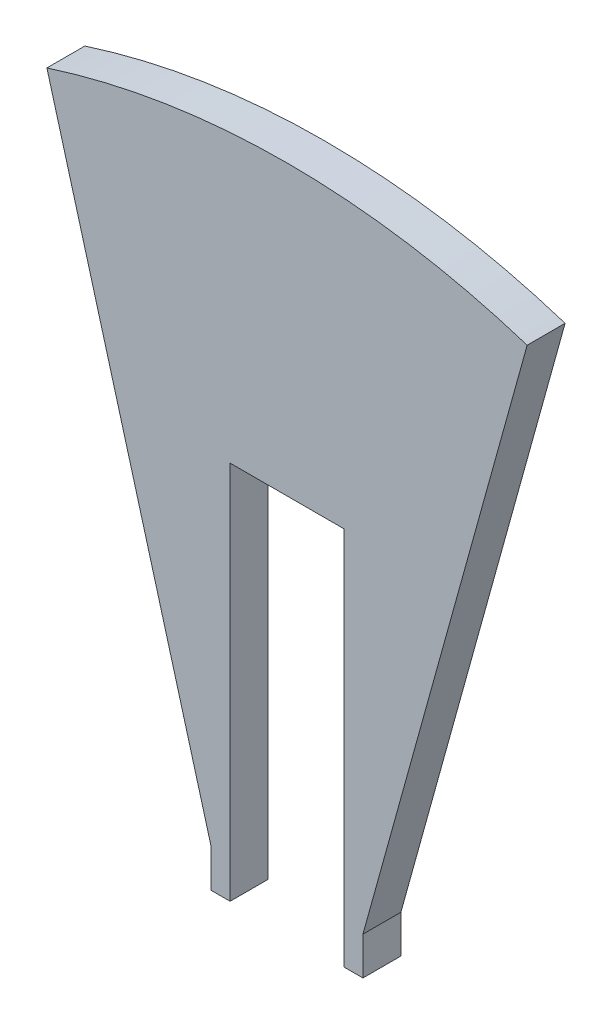
from build123d import *

# Parameters (mm, degrees)
BOSS_EXTRUDE1_DEPTH = 5
SKETCH2_W           = 30
SKETCH2_H           = 200
CUT_EXTRUDE1_DEPTH  = 10


with BuildPart() as part:
    # Sketch1 → Boss-Extrude1 (new, symmetric)
    with BuildSketch(Plane.XY):
        with BuildLine():
            Line((-63.274211694, 196.041766301), (-20, 40))
            Line((-20, 40), (-20, 30))
            Line((-20, 30), (20, 30))
            Line((20, 30), (20, 40))
            Line((20, 40), (63.274211694, 196.041766301))
            ThreePointArc((63.274211694, 196.041766301), (0, 206), (-63.274211694, 196.041766301))
        make_face()
    extrude(amount=BOSS_EXTRUDE1_DEPTH, both=True)

    # Sketch2 → Cut-Extrude1 (cut)
    with BuildSketch(Plane.XY.offset(5)):
        with Locations((0, 30)):
            Rectangle(SKETCH2_W, SKETCH2_H)
    extrude(amount=-CUT_EXTRUDE1_DEPTH, mode=Mode.SUBTRACT)


solid = part.part
